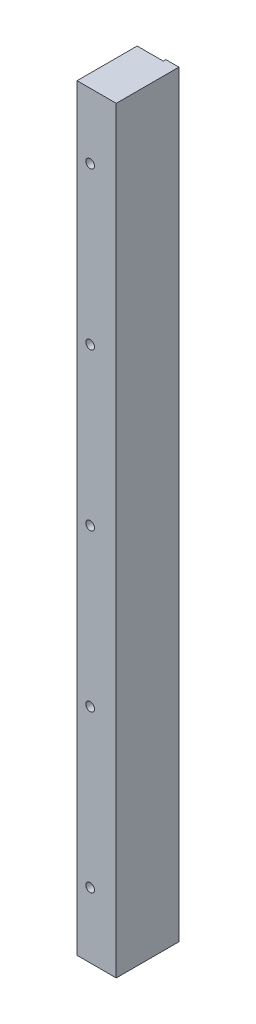
from build123d import *

# Parameters (mm, degrees)
SKETCH_1_W                = 30
SKETCH_1_H                = 580
EXTRUDE_1_DEPTH           = 48
SKETCH_2_W                = 20
SKETCH_2_H                = 580
CUT_EXTRUDE_1_DEPTH       = 2
PATTERN_LINEAR_1_COUNT    = 10
PATTERN_LINEAR_1_PITCH    = 60
HOLE_WIZARD_1_D           = 6.6
HOLE_WIZARD_1_CBORE_D     = 11
HOLE_WIZARD_1_CBORE_DEPTH = 6.8
PATTERN_LINEAR_2_COUNT    = 5
PATTERN_LINEAR_2_PITCH    = 120


with BuildPart() as part:
    # 草图1 → 凸台-拉伸1 (new body)
    with BuildSketch(Plane.XY):
        Rectangle(SKETCH_1_W, SKETCH_1_H)
    extrude(amount=EXTRUDE_1_DEPTH)

    # 草图2 → 切除-拉伸1 (cut)
    with BuildSketch(Plane(origin=(0, 0, 0), x_dir=(-1, 0, 0), z_dir=(0, 0, -1))):
        with Locations((5, 0)):
            Rectangle(SKETCH_2_W, SKETCH_2_H)
    extrude(amount=-CUT_EXTRUDE_1_DEPTH, mode=Mode.SUBTRACT)

    # 草图4 → M5 螺纹孔1 (revolve, cut)
    with BuildSketch(Plane(origin=(-5, 270, 2), x_dir=(0, 1, 0), z_dir=(1, 0, 0))):
        Polygon((0, 0), (0, 13.6618073), (2.1, 12.4), (2.1, 0), align=None)
    hole_wizard_m5_1 = revolve(axis=Axis((-5, 270, -4.35), (0, 0, 1)), mode=Mode.SUBTRACT)

    # 阵列(线性)1: M5 螺纹孔1 ×10
    with Locations(*[(0, -i * PATTERN_LINEAR_1_PITCH, 0) for i in range(1, PATTERN_LINEAR_1_COUNT)]):
        add(hole_wizard_m5_1, mode=Mode.SUBTRACT)

    # 打孔尺寸(%根据)内六角圆柱头螺钉的类型1 (through all)
    with Locations(Plane(origin=(0, 0, 2), x_dir=(-1, 0, 0), z_dir=(0, 0, -1))):
        with Locations((5, 240)):
            hole_wizard_1 = CounterBoreHole(HOLE_WIZARD_1_D / 2, HOLE_WIZARD_1_CBORE_D / 2, HOLE_WIZARD_1_CBORE_DEPTH)

    # 阵列(线性)2: 打孔尺寸(%根据)内六角圆柱头螺钉的类型1 ×5
    with Locations(*[(0, -i * PATTERN_LINEAR_2_PITCH, 0) for i in range(1, PATTERN_LINEAR_2_COUNT)]):
        add(hole_wizard_1, mode=Mode.SUBTRACT)


solid = part.part
